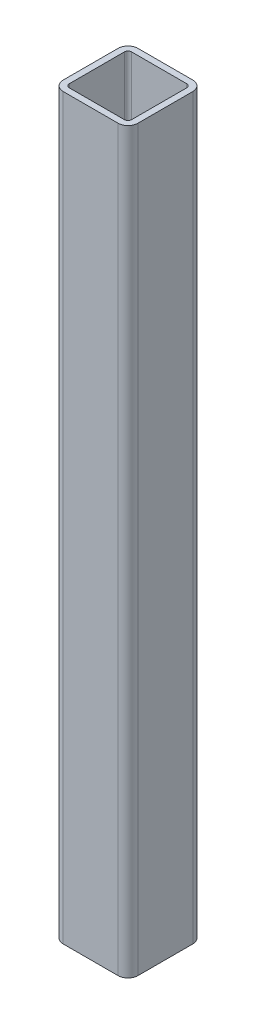
SolidWorks part; units mm, degrees
material "XRAAT"
ref_plane "前视基准面" through (0, 0, 0) normal (0, 0, 1) x (1, 0, 0)
ref_plane "上视基准面" through (0, 0, 0) normal (0, 1, 0) x (1, 0, 0)
ref_plane "右视基准面" through (0, 0, 0) normal (1, 0, 0) x (0, 0, -1)
sketch "草图1" plane through (0, 0, 0) normal (0, 0, 1) x (1, 0, 0)
  line L0 (0, 0) -> (0, 1185)
  dimension "D1" = 1185
other "结构用冷弯空心方钢(gb t6728-2002) 120×120×10(1)"
ref_plane "基准面1" through (0, 0, 0) normal (0, 1, 0) x (-1, 0, 0)
sketch "Sketch12" plane through (0, 0, 0) normal (0, 1, 0) x (-1, 0, 0)
  line L0 (-44, -50) -> (44, -50)
  line L1 (-50, -44) -> (-50, 44)
  line L2 (44, 50) -> (-44, 50)
  line L3 (50, 44) -> (50, -44)
  line L4 (-44, -60) -> (44, -60)
  line L5 (-60, -44) -> (-60, 44)
  line L6 (44, 60) -> (-44, 60)
  line L7 (60, 44) -> (60, -44)
  arc A0 (60, 44) -> (44, 60) centre (44, 44) ccw
  arc A1 (44, -60) -> (60, -44) centre (44, -44) ccw
  arc A2 (-60, -44) -> (-44, -60) centre (-44, -44) ccw
  arc A3 (-44, 60) -> (-60, 44) centre (-44, 44) ccw
  arc A4 (-44, 50) -> (-50, 44) centre (-44, 44) ccw
  arc A5 (50, 44) -> (44, 50) centre (44, 44) ccw
  arc A6 (44, -50) -> (50, -44) centre (44, -44) ccw
  arc A7 (-50, -44) -> (-44, -50) centre (-44, -44) ccw
  point P0 (-60, 0)
  point P1 (60, 0)
  point P2 (0, 60)
  point P3 (0, -60)
  point P4 (0, 0)
  point P5 (-60, -60)
  point P6 (60, -60)
  point P7 (60, 60)
  point P8 (-60, 60)
  point P33 (0, 0)
  dimension "D1" = 16
  dimension "D2" = 120
  dimension "D3" = 10
